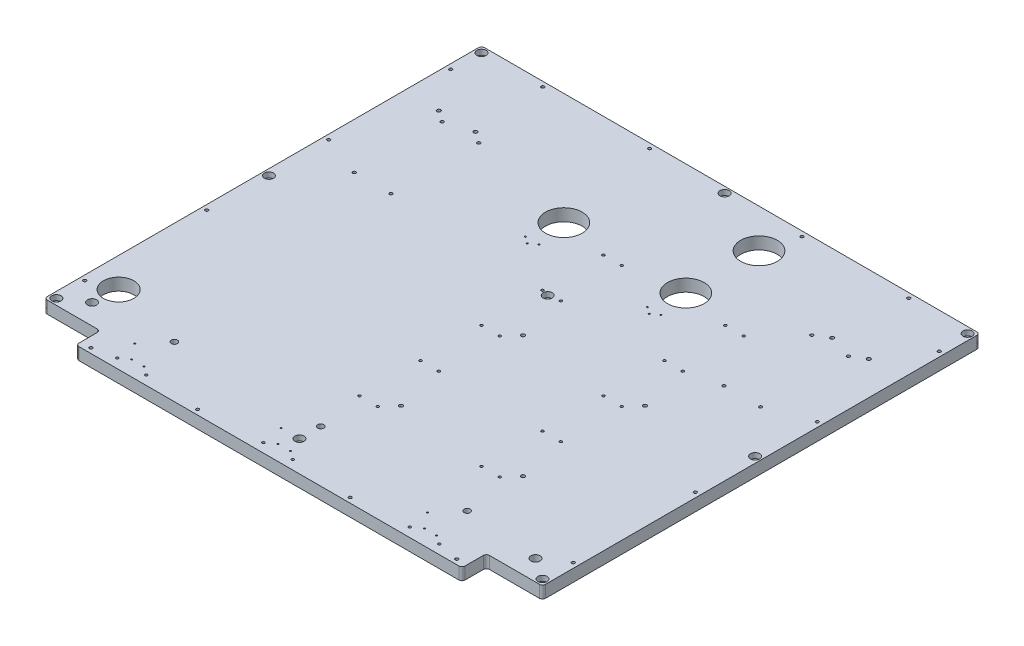
from build123d import *

# Parameters (mm, degrees)
SKETCH_1_W                   = 850
SKETCH_1_H                   = 750
EXTRUDE_1_DEPTH              = 20
CUT_EXTRUDE_13_REACH         = 569.142
SKETCH_48_R                  = 30
CUT_EXTRUDE_12_REACH         = 569.142
SKETCH_47_R                  = 25
SKETCH_37_W                  = 850
SKETCH_37_H                  = 750
SKETCH_37_W_2                = 817
SKETCH_37_H_2                = 717
CUT_EXTRUDE_10_DEPTH         = 568.141957538
SKETCH_38_W                  = 633
SKETCH_38_H                  = 40
EXTRUDE_2_DEPTH              = 20
CUT_EXTRUDE_14_REACH         = 573.029
SKETCH_56_R                  = 7.5
HOLE_WIZARD_M8_2_D           = 9
HOLE_WIZARD_M8_2_CBORE_D     = 15
HOLE_WIZARD_M8_2_CBORE_DEPTH = 8.6
HOLE_WIZARD_M5_2_D           = 4.2
HOLE_WIZARD_M5_2_DEPTH       = 12.4
HOLE_WIZARD_M5_2_TIP         = 1.2618073
HOLE_WIZARD_M3_3_D           = 2.5
HOLE_WIZARD_M3_3_DEPTH       = 7.5
HOLE_WIZARD_M3_3_TIP         = 0.751075774
HOLE_WIZARD_10_0_10_1_D      = 10
HOLE_WIZARD_M6_3_D           = 5
HOLE_WIZARD_M6_4_D           = 5
HOLE_WIZARD_M5_3_D           = 4.2
PATTERN_LINEAR_4_COUNT       = 2
PATTERN_LINEAR_4_PITCH       = 30
PATTERN_LINEAR_4_COUNT_DIR2  = 5
PATTERN_LINEAR_4_PITCH_DIR2  = 100
PATTERN_LINEAR_5_COUNT       = 2
PATTERN_LINEAR_5_PITCH       = 200
PATTERN_LINEAR_5_COPY_1_D    = 4.2
PATTERN_LINEAR_5_COPY_2_D    = 4.2
PATTERN_LINEAR_5_COPY_3_D    = 4.2
PATTERN_LINEAR_5_COPY_4_D    = 4.2
PATTERN_LINEAR_5_COPY_5_D    = 4.2
PATTERN_LINEAR_5_COPY_6_D    = 4.2
PATTERN_LINEAR_5_COPY_7_D    = 4.2
PATTERN_LINEAR_5_COPY_8_D    = 4.2
PATTERN_LINEAR_5_COPY_9_D    = 4.2
HOLE_WIZARD_6_0_6_1_D        = 6
HOLE_WIZARD_6_0_6_1_DEPTH    = 15
HOLE_WIZARD_6_0_6_1_TIP      = 1.802581857
HOLE_WIZARD_6_0_6_2_D        = 6
HOLE_WIZARD_6_0_6_2_DEPTH    = 10
HOLE_WIZARD_6_0_6_2_TIP      = 1.802581857
HOLE_WIZARD_M3_4_D           = 2.5
HOLE_WIZARD_M3_4_DEPTH       = 7.5
HOLE_WIZARD_M3_4_TIP         = 0.751075774
FILLET_1_R                   = 5


with BuildPart() as part:
    # 草图1 → 凸台-拉伸1 (new body)
    with BuildSketch(Plane(origin=(0, 0, 0), x_dir=(1, 0, 0), z_dir=(0, 1, 0))):
        Rectangle(SKETCH_1_W, SKETCH_1_H)
    extrude(amount=EXTRUDE_1_DEPTH)

    # 草图48 → 切除-拉伸13 (cut, up to next)
    with BuildSketch(Plane(origin=(0, 20, 0), x_dir=(1, 0, 0), z_dir=(0, 1, 0)), mode=Mode.PRIVATE) as cut_extrude_13_sk1:
        with Locations(Location((-90, 175, 0), (0, 0, 270))):
            Circle(SKETCH_48_R)
    cut_extrude_13_tool1 = extrude(cut_extrude_13_sk1.sketch, amount=-CUT_EXTRUDE_13_REACH, mode=Mode.PRIVATE) & part.part
    # 草图48 → 切除-拉伸13 (cut, up to next)
    with BuildSketch(Plane(origin=(0, 20, 0), x_dir=(1, 0, 0), z_dir=(0, 1, 0)), mode=Mode.PRIVATE) as cut_extrude_13_sk2:
        with Locations(Location((110, 175, 0), (0, 0, 270))):
            Circle(SKETCH_48_R)
    cut_extrude_13_tool2 = extrude(cut_extrude_13_sk2.sketch, amount=-CUT_EXTRUDE_13_REACH, mode=Mode.PRIVATE) & part.part
    # 草图48 → 切除-拉伸13 (cut, up to next)
    with BuildSketch(Plane(origin=(0, 20, 0), x_dir=(1, 0, 0), z_dir=(0, 1, 0)), mode=Mode.PRIVATE) as cut_extrude_13_sk3:
        with Locations(Location((110, 295, 0), (0, 0, 270))):
            Circle(SKETCH_48_R)
    cut_extrude_13_tool3 = extrude(cut_extrude_13_sk3.sketch, amount=-CUT_EXTRUDE_13_REACH, mode=Mode.PRIVATE) & part.part
    add(cut_extrude_13_tool1.solids().sort_by_distance((-90, 20, -175))[0], mode=Mode.SUBTRACT)
    add(cut_extrude_13_tool2.solids().sort_by_distance((110, 20, -175))[0], mode=Mode.SUBTRACT)
    add(cut_extrude_13_tool3.solids().sort_by_distance((110, 20, -295))[0], mode=Mode.SUBTRACT)

    # 草图47 → 切除-拉伸12 (cut, up to next)
    with BuildSketch(Plane(origin=(0, 20, 0), x_dir=(1, 0, 0), z_dir=(0, 1, 0)), mode=Mode.PRIVATE) as cut_extrude_12_sk1:
        with Locations(Location((-360, -285, 0), (0, 0, 270))):
            Circle(SKETCH_47_R)
    cut_extrude_12_tool1 = extrude(cut_extrude_12_sk1.sketch, amount=-CUT_EXTRUDE_12_REACH, mode=Mode.PRIVATE) & part.part
    add(cut_extrude_12_tool1.solids().sort_by_distance((-360, 20, 285))[0], mode=Mode.SUBTRACT)

    # 草图37 → 切除-拉伸10 (cut, through all)
    with BuildSketch(Plane(origin=(0, 20, 0), x_dir=(-1, 0, 0), z_dir=(0, -1, 0))):
        Rectangle(SKETCH_37_W, SKETCH_37_H)
        Rectangle(SKETCH_37_W_2, SKETCH_37_H_2, mode=Mode.SUBTRACT)
    extrude(amount=CUT_EXTRUDE_10_DEPTH, mode=Mode.SUBTRACT)

    # 草图38 → 凸台-拉伸2 (add)
    with BuildSketch(Plane(origin=(0, 20, 0), x_dir=(1, 0, 0), z_dir=(0, 1, 0))):
        with Locations((0, -378.5)):
            Rectangle(SKETCH_38_W, SKETCH_38_H)
    extrude(amount=-EXTRUDE_2_DEPTH)

    # 草图56 → 切除-拉伸14 (cut, up to next)
    with BuildSketch(Plane(origin=(0, 20, 0), x_dir=(1, 0, 0), z_dir=(0, 1, 0)), mode=Mode.PRIVATE) as cut_extrude_14_sk1:
        with Locations(Location((-363.5, -325, 0), (0, 0, 270))):
            Circle(SKETCH_56_R)
    cut_extrude_14_tool1 = extrude(cut_extrude_14_sk1.sketch, amount=-CUT_EXTRUDE_14_REACH, mode=Mode.PRIVATE) & part.part
    # 草图56 → 切除-拉伸14 (cut, up to next)
    with BuildSketch(Plane(origin=(0, 20, 0), x_dir=(1, 0, 0), z_dir=(0, 1, 0)), mode=Mode.PRIVATE) as cut_extrude_14_sk2:
        with Locations(Location((363.5, -325, 0), (0, 0, 270))):
            Circle(SKETCH_56_R)
    cut_extrude_14_tool2 = extrude(cut_extrude_14_sk2.sketch, amount=-CUT_EXTRUDE_14_REACH, mode=Mode.PRIVATE) & part.part
    add(cut_extrude_14_tool1.solids().sort_by_distance((-363.5, 20, 325))[0], mode=Mode.SUBTRACT)
    add(cut_extrude_14_tool2.solids().sort_by_distance((363.5, 20, 325))[0], mode=Mode.SUBTRACT)

    # M8 六角凹头螺钉的柱形沉头孔2 (through all)
    with Locations(Plane(origin=(0, 20, 0), x_dir=(1, 0, 0), z_dir=(0, 1, 0))):
        with Locations((-398.5, 348.5), (-398.5, 0), (-398.5, -348.5), (0, -348.5), (398.5, -348.5), (398.5, 0), (398.5, 348.5), (0, 348.5), (0, 58.5)):
            CounterBoreHole(HOLE_WIZARD_M8_2_D / 2, HOLE_WIZARD_M8_2_CBORE_D / 2, HOLE_WIZARD_M8_2_CBORE_DEPTH)

    # M5 螺纹孔2
    with Locations(Plane(origin=(0.65261799, 20, 1.972370981), x_dir=(-1, 0, 0), z_dir=(0, 1, 0))):
        with Locations((-215.34738201, 381.527629019), (-263.34738201, 381.527629019), (24.65261799, 381.527629019), (-23.34738201, 381.527629019), (264.65261799, 381.527629019), (216.65261799, 381.527629019)):
            Hole(HOLE_WIZARD_M5_2_D / 2, depth=HOLE_WIZARD_M5_2_DEPTH)
            with Locations((0, 0, -(HOLE_WIZARD_M5_2_DEPTH + HOLE_WIZARD_M5_2_TIP / 2))):  # 118° drill point
                Cone(0, HOLE_WIZARD_M5_2_D / 2, HOLE_WIZARD_M5_2_TIP, mode=Mode.SUBTRACT)

    # M3 螺纹孔3
    with Locations(Plane(origin=(-240.455895113, 20, 219.833750801), x_dir=(-1, 0, 0), z_dir=(0, 1, 0))):
        with Locations((9.544104887, 153.666249199), (-10.455895113, 153.666249199), (-230.455895113, 153.666249199), (-250.455895113, 153.666249199), (-470.455895113, 153.666249199), (-490.455895113, 153.666249199), (29.544104887, 128.666249199), (-210.455895113, 128.666249199), (-450.455895113, 128.666249199)):
            Hole(HOLE_WIZARD_M3_3_D / 2, depth=HOLE_WIZARD_M3_3_DEPTH)
            with Locations((0, 0, -(HOLE_WIZARD_M3_3_DEPTH + HOLE_WIZARD_M3_3_TIP / 2))):  # 118° drill point
                Cone(0, HOLE_WIZARD_M3_3_D / 2, HOLE_WIZARD_M3_3_TIP, mode=Mode.SUBTRACT)

    # Ø10.0 (10) 直径孔1 (through all)
    with Locations(Plane(origin=(0, 20, 0), x_dir=(1, 0, 0), z_dir=(0, 1, 0))):
        with Locations((-240, -313.5), (0, -313.5), (240, -313.5)):
            Hole(HOLE_WIZARD_10_0_10_1_D / 2)

    # M6 螺纹孔3 (through all)
    with Locations(Plane(origin=(0, 20, 0), x_dir=(1, 0, 0), z_dir=(0, 1, 0))):
        with Locations((-300, 350.5), (-125, 350.5), (125, 350.5), (300, 350.5), (-300, -390.5), (-125, -390.5), (125, -390.5), (300, -390.5), (-400.5, 300), (-400.5, 100), (-400.5, -100), (-400.5, -300), (400.5, 300), (400.5, 100), (400.5, -100), (400.5, -300)):
            Hole(HOLE_WIZARD_M6_3_D / 2)

    # M6 螺纹孔4 (through all)
    with Locations(Plane(origin=(0, 20, 0), x_dir=(1, 0, 0), z_dir=(0, 1, 0))):
        with Locations((333, 218.5), (273, 218.5), (273, 74.5), (333, 74.5), (-333, 218.5), (-273, 218.5), (-333, 74.5), (-273, 74.5)):
            Hole(HOLE_WIZARD_M6_4_D / 2)

    # M5 螺纹孔3 (through all)
    with Locations(Plane(origin=(0, 20, 0), x_dir=(1, 0, 0), z_dir=(0, 1, 0))):
        with Locations((218.5, -238.5)):
            hole_wizard_m5_3 = Hole(HOLE_WIZARD_M5_3_D / 2)

    # 阵列(线性)4: Hole Wizard M5 _3 2 × 5
    with Locations(*[(-i * PATTERN_LINEAR_4_PITCH, 0, -j * PATTERN_LINEAR_4_PITCH_DIR2) for i in range(PATTERN_LINEAR_4_COUNT) for j in range(PATTERN_LINEAR_4_COUNT_DIR2) if (i, j) != (0, 0)]):
        add(hole_wizard_m5_3, mode=Mode.SUBTRACT)

    # 阵列(线性)5: M5 螺纹孔3 ×2
    with Locations(*[(-i * PATTERN_LINEAR_5_PITCH, 0, 0) for i in range(1, PATTERN_LINEAR_5_COUNT)]):
        add(hole_wizard_m5_3, mode=Mode.SUBTRACT)

    # 阵列(线性)5 copy 1 (through all)
    with Locations(Plane(origin=(-200, 20, -100), x_dir=(1, 0, 0), z_dir=(0, 1, 0))):
        with Locations((218.5, -238.5)):
            Hole(PATTERN_LINEAR_5_COPY_1_D / 2)

    # 阵列(线性)5 copy 2 (through all)
    with Locations(Plane(origin=(-200, 20, -200), x_dir=(1, 0, 0), z_dir=(0, 1, 0))):
        with Locations((218.5, -238.5)):
            Hole(PATTERN_LINEAR_5_COPY_2_D / 2)

    # 阵列(线性)5 copy 3 (through all)
    with Locations(Plane(origin=(-200, 20, -300), x_dir=(1, 0, 0), z_dir=(0, 1, 0))):
        with Locations((218.5, -238.5)):
            Hole(PATTERN_LINEAR_5_COPY_3_D / 2)

    # 阵列(线性)5 copy 4 (through all)
    with Locations(Plane(origin=(-200, 20, -400), x_dir=(1, 0, 0), z_dir=(0, 1, 0))):
        with Locations((218.5, -238.5)):
            Hole(PATTERN_LINEAR_5_COPY_4_D / 2)

    # 阵列(线性)5 copy 5 (through all)
    with Locations(Plane(origin=(-230, 20, 0), x_dir=(1, 0, 0), z_dir=(0, 1, 0))):
        with Locations((218.5, -238.5)):
            Hole(PATTERN_LINEAR_5_COPY_5_D / 2)

    # 阵列(线性)5 copy 6 (through all)
    with Locations(Plane(origin=(-230, 20, -100), x_dir=(1, 0, 0), z_dir=(0, 1, 0))):
        with Locations((218.5, -238.5)):
            Hole(PATTERN_LINEAR_5_COPY_6_D / 2)

    # 阵列(线性)5 copy 7 (through all)
    with Locations(Plane(origin=(-230, 20, -200), x_dir=(1, 0, 0), z_dir=(0, 1, 0))):
        with Locations((218.5, -238.5)):
            Hole(PATTERN_LINEAR_5_COPY_7_D / 2)

    # 阵列(线性)5 copy 8 (through all)
    with Locations(Plane(origin=(-230, 20, -300), x_dir=(1, 0, 0), z_dir=(0, 1, 0))):
        with Locations((218.5, -238.5)):
            Hole(PATTERN_LINEAR_5_COPY_8_D / 2)

    # 阵列(线性)5 copy 9 (through all)
    with Locations(Plane(origin=(-230, 20, -400), x_dir=(1, 0, 0), z_dir=(0, 1, 0))):
        with Locations((218.5, -238.5)):
            Hole(PATTERN_LINEAR_5_COPY_9_D / 2)

    # Ø6.0 (6) 直径孔1
    with Locations(Plane(origin=(0, 20, 0), x_dir=(1, 0, 0), z_dir=(0, 1, 0))):
        with Locations((236.5, -18.5), (236.5, -218.5), (36.5, -18.5), (36.5, -218.5)):
            Hole(HOLE_WIZARD_6_0_6_1_D / 2, depth=HOLE_WIZARD_6_0_6_1_DEPTH)
            with Locations((0, 0, -(HOLE_WIZARD_6_0_6_1_DEPTH + HOLE_WIZARD_6_0_6_1_TIP / 2))):  # 118° drill point
                Cone(0, HOLE_WIZARD_6_0_6_1_D / 2, HOLE_WIZARD_6_0_6_1_TIP, mode=Mode.SUBTRACT)

    # Ø6.0 (6) 直径孔2
    with Locations(Plane(origin=(0, 20, 0), x_dir=(1, 0, 0), z_dir=(0, 1, 0))):
        with Locations((-351.5, 231.5), (-291.5, 231.5), (293.5, 231.5), (353.5, 231.5)):
            Hole(HOLE_WIZARD_6_0_6_2_D / 2, depth=HOLE_WIZARD_6_0_6_2_DEPTH)
            with Locations((0, 0, -(HOLE_WIZARD_6_0_6_2_DEPTH + HOLE_WIZARD_6_0_6_2_TIP / 2))):  # 118° drill point
                Cone(0, HOLE_WIZARD_6_0_6_2_D / 2, HOLE_WIZARD_6_0_6_2_TIP, mode=Mode.SUBTRACT)

    # M3 螺纹孔4
    with Locations(Plane(origin=(0, 20, 0), x_dir=(1, 0, 0), z_dir=(0, 1, 0))):
        with Locations((98.5, 123.5), (120.5, 123.5), (109.5, 115.5), (-101.5, 123.5), (-79.5, 123.5), (-90.5, 115.5)):
            Hole(HOLE_WIZARD_M3_4_D / 2, depth=HOLE_WIZARD_M3_4_DEPTH)
            with Locations((0, 0, -(HOLE_WIZARD_M3_4_DEPTH + HOLE_WIZARD_M3_4_TIP / 2))):  # 118° drill point
                Cone(0, HOLE_WIZARD_M3_4_D / 2, HOLE_WIZARD_M3_4_TIP, mode=Mode.SUBTRACT)

    # 圆角1
    fillet_1_edges = [part.edges().sort_by_distance(p)[0] for p in [
        (-408.5, 10, 358.5),
        (408.5, 10, 358.5),
        (408.5, 10, -358.5),
        (-408.5, 10, -358.5),
        (-316.5, 10, 358.5),
        (-316.5, 10, 398.5),
        (316.5, 10, 398.5),
        (316.5, 10, 358.5),
    ]]
    fillet(fillet_1_edges, radius=FILLET_1_R)


solid = part.part
